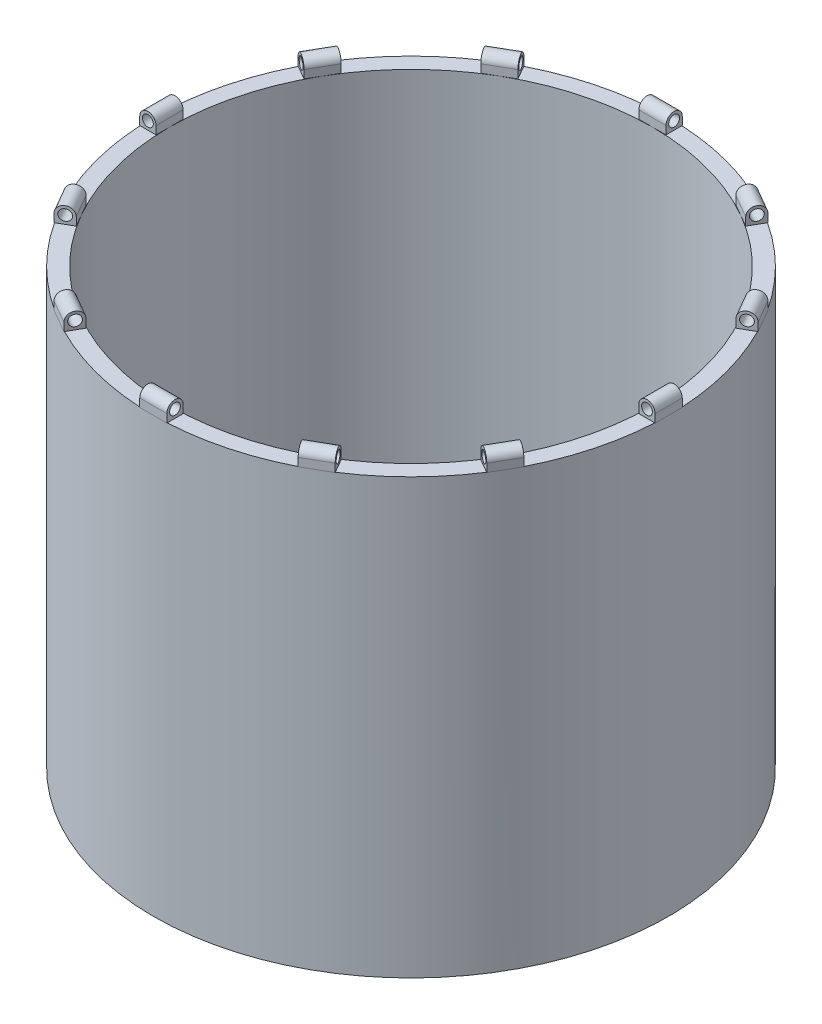
SolidWorks part; units mm, degrees
ref_plane "前视基准面" through (0, 0, 0) normal (0, 0, 1) x (1, 0, 0)
ref_plane "上视基准面" through (0, 0, 0) normal (0, 1, 0) x (1, 0, 0)
ref_plane "右视基准面" through (0, 0, 0) normal (1, 0, 0) x (0, 0, -1)
sketch "草图1" plane through (0, 0, 0) normal (0, 1, 0) x (1, 0, 0)
  circle A0 centre (0, 0) radius 47.5
  circle A1 centre (0, 0) radius 44.5
  dimension "D1" = 95
  dimension "D2" = 89
extrude "凸台-拉伸1" add sketch "草图1" along normal blind 80
sketch "草图2" plane through (0, 0, 0) normal (1, 0, 0) x (0, 0, -1)
  line L0 (47.5, 80) -> (-47.5, 80) construction
  line L1 (-47.5, 80) -> (-47.5, 0) construction
  line L2 (-47.5, 81.5) -> (-47.5, 80)
  line L3 (-47.5, 80) -> (-44.5, 80)
  line L4 (-44.5, 80) -> (-44.5, 81.5)
  circle A0 centre (-46, 81.5) radius 1.5
  circle A1 centre (-46, 81.5) radius 1
  dimension "D1" = 3
  dimension "D2" = 2
  dimension "D3" = 1.5
  dimension "D4" = 1.5
extrude "凸台-拉伸3" add sketch "草图2" along normal mid plane 5 contours A0 L2 L3 | A0 L3 L4 | A0 A1
pattern_circular "阵列(圆周)1" count 12 over 360 about axis through (0, 0, 0) along (0, 1, 0) of "凸台-拉伸3"
